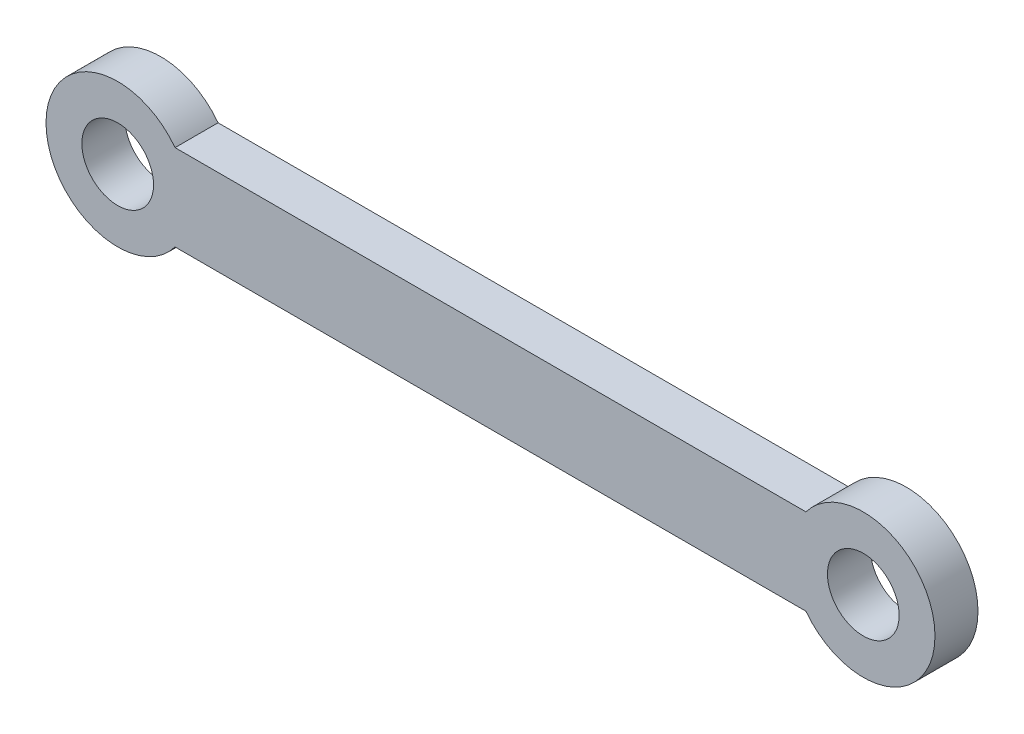
from build123d import *

# Parameters (mm, degrees)
SKETCH1_R           = 2.5
BOSS_EXTRUDE1_DEPTH = 3


with BuildPart() as part:
    # Sketch1 → Boss-Extrude1 (new body)
    with BuildSketch(Plane.XY):
        with BuildLine():
            Line((4, 3), (48, 3))
            ThreePointArc((48, 3), (57, 0), (48, -3))
            Line((48, -3), (4, -3))
            ThreePointArc((4, -3), (-5, 0), (4, 3))
        make_face()
        Circle(SKETCH1_R, mode=Mode.SUBTRACT)
        with Locations((52, 0)):
            Circle(SKETCH1_R, mode=Mode.SUBTRACT)
    extrude(amount=BOSS_EXTRUDE1_DEPTH)


solid = part.part
